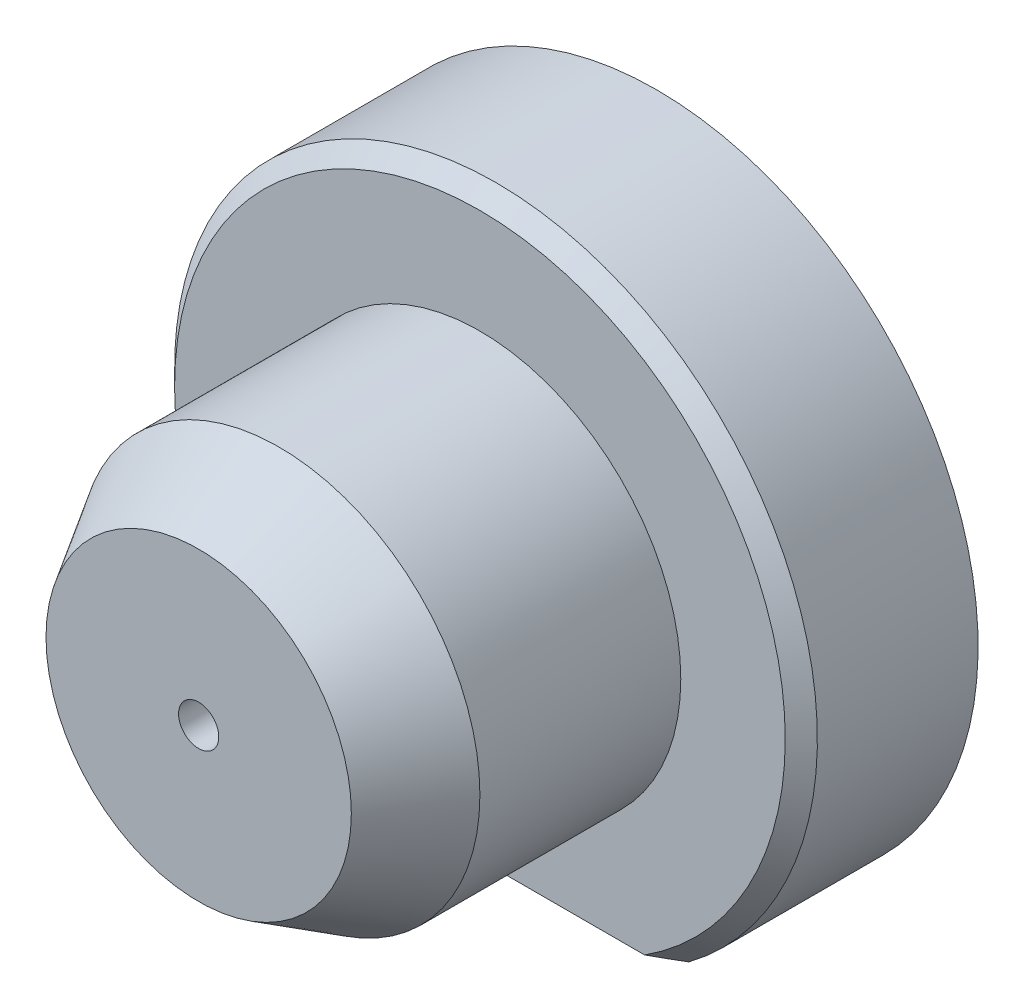
SolidWorks part; units mm, degrees
material "SUJ2"
ref_plane "Front Plane" through (0, 0, 0) normal (0, 0, 1) x (1, 0, 0)
ref_plane "Top Plane" through (0, 0, 0) normal (0, 1, 0) x (1, 0, 0)
ref_plane "Right Plane" through (0, 0, 0) normal (1, 0, 0) x (0, 0, -1)
sketch "Sketch1" plane through (0, 0, 0) normal (0, 0, 1) x (1, 0, 0)
  circle A0 centre (0, 0) radius 25
  dimension "D1" = 50
extrude "Boss-Extrude1" add sketch "Sketch1" along normal blind 35
chamfer "Chamfer1" distance 10 distance2 6 1 edges at (25, 0, 35)
sketch "Sketch2" plane through (0, 0, 0) normal (0, 0, -1) x (-1, 0, 0)
  circle A0 centre (0, 0) radius 40
  dimension "D1" = 80
extrude "Boss-Extrude2" add sketch "Sketch2" along normal blind 22
sketch "Sketch3" plane through (0, 0, 0) normal (1, 0, 0) x (0, 0, -1)
  line L0 (0, -40) -> (22, -40) construction
  line L1 (-68, -62) -> (22, -62)
  line L2 (-68, -62) -> (-68, -32)
  line L3 (-68, -32) -> (22, -32)
  line L4 (22, -62) -> (22, -32)
  line L5 (22, -40) -> (22, 40) construction
  dimension "D1" = 8
  dimension "D2" = 90
  dimension "D3" = 30
extrude "Cut-Extrude1" cut sketch "Sketch3" against normal mid plane 60
chamfer "Chamfer2" distance 2 angle 45 1 edges at (0, 40, 0)
hole_wizard "M6 Tapped Hole1" positions "Sketch8" profile "Sketch7" tap size "M6" standard "GB" end condition through all
sketch "Sketch8" plane through (0, 0, -22) normal (0, 0, -1) x (-1, 0, 0)
  point P0 (0, 0)
sketch "Sketch7" plane through (0, 0, -22) normal (1, 0, 0) x (0, 1, 0)
  line L0 (0, 0) -> (0, 57)
  line L1 (0, 57) -> (2.5, 57)
  line L2 (2.5, 57) -> (2.5, 0)
  line L5 (2.5, 0) -> (0, 0)
  line L11 (0, -6.35) -> (0, 107.95) construction
  dimension "通孔螺纹孔钻头直径" = 5
  dimension "通孔螺纹孔钻头深度" = 57
cosmetic thread "Hole thread1" parameters "D2"=6
